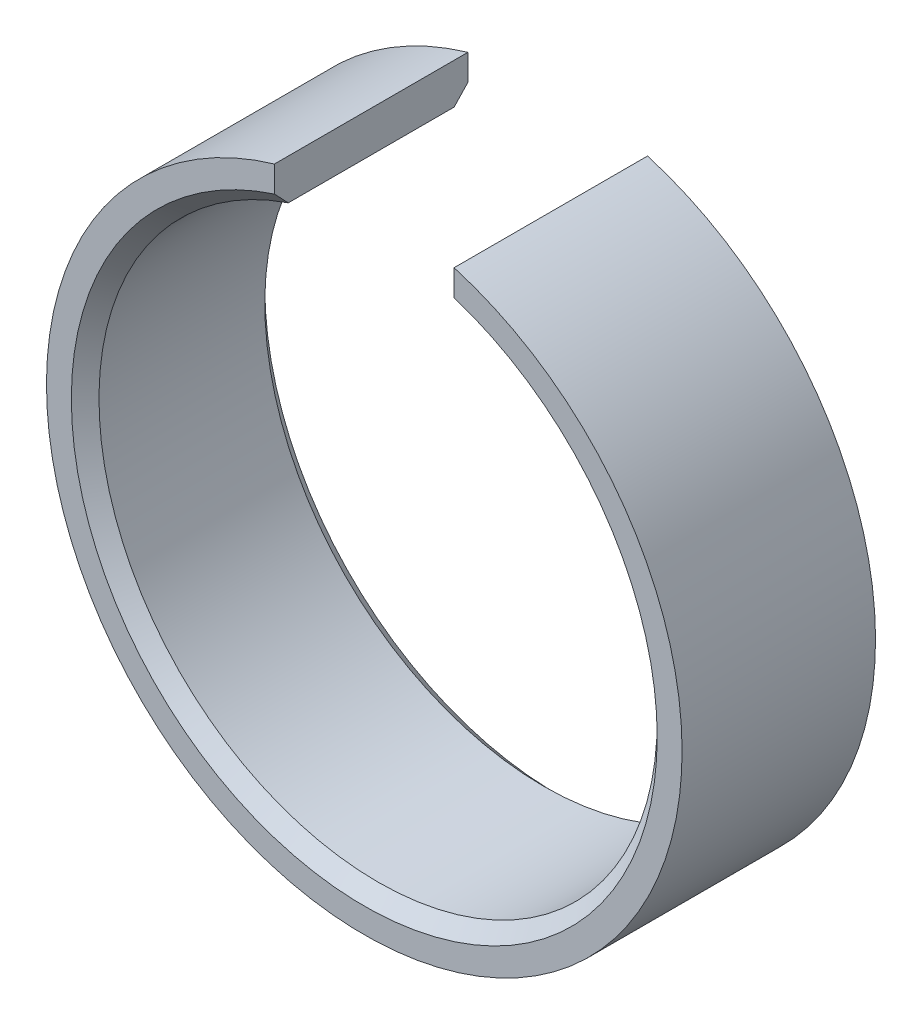
from build123d import *

# Parameters (mm, degrees)
SKETCH1_R           = 11.5
SKETCH1_R_2         = 10.1
BOSS_EXTRUDE1_DEPTH = 7
SKETCH2_W           = 6.5
SKETCH2_H           = 15
CUT_EXTRUDE1_DEPTH  = 18.70593121
CHAMFER1_SIZE       = 0.5


with BuildPart() as part:
    # Sketch1 → Boss-Extrude1 (new body)
    with BuildSketch(Plane.XY):
        Circle(SKETCH1_R)
        Circle(SKETCH1_R_2, mode=Mode.SUBTRACT)
    extrude(amount=BOSS_EXTRUDE1_DEPTH)

    # Sketch2 → Cut-Extrude1 (cut, through all)
    with BuildSketch(Plane.XY.offset(7)):
        with Locations((0, 7.5)):
            Rectangle(SKETCH2_W, SKETCH2_H)
    extrude(amount=-CUT_EXTRUDE1_DEPTH, mode=Mode.SUBTRACT)

    # Chamfer1
    chamfer1_edges = [part.edges().sort_by_distance(p)[0] for p in [
        (0, -10.1, 0),
        (0, -10.1, 7),
    ]]
    chamfer(chamfer1_edges, length=CHAMFER1_SIZE)


solid = part.part
